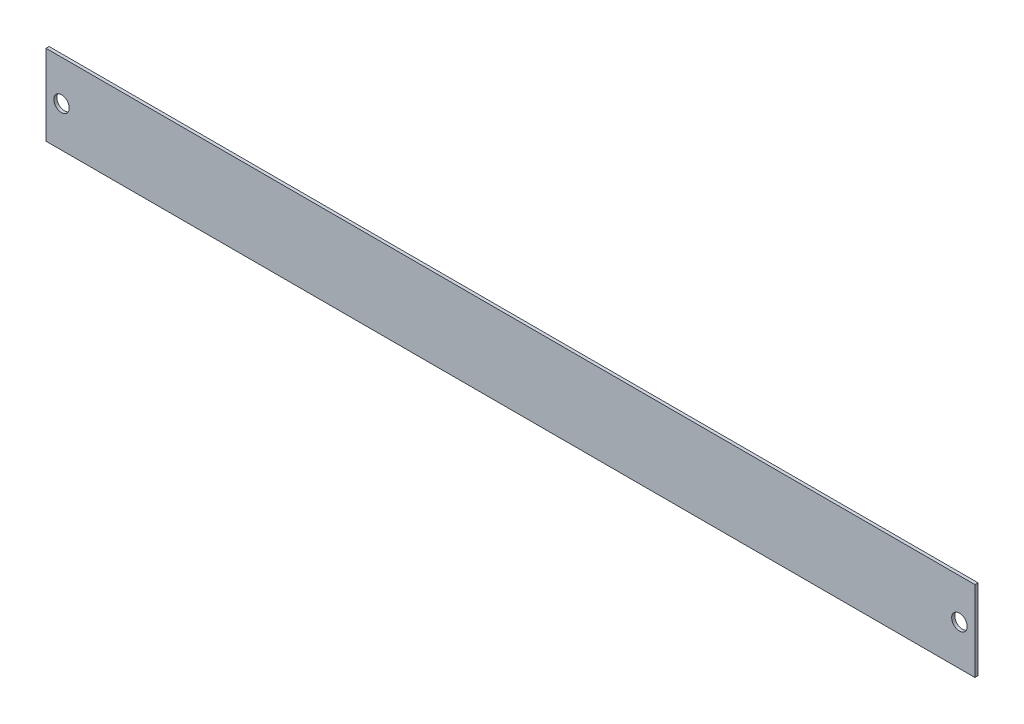
from build123d import *

# Parameters (mm, degrees)
SKETCH_1_W                = 300
SKETCH_1_H                = 26
EXTRUDE_1_DEPTH           = 1
HOLE_WIZARD_5_0_5_1_D     = 5
HOLE_WIZARD_5_0_5_1_DEPTH = 5
HOLE_WIZARD_5_0_5_1_TIP   = 1.502151548


with BuildPart() as part:
    # 草图1 → 凸台-拉伸1 (new body)
    with BuildSketch(Plane.XY):
        with Locations((0, 13)):
            Rectangle(SKETCH_1_W, SKETCH_1_H)
    extrude(amount=EXTRUDE_1_DEPTH)

    # Ø5.0 (5) 直径孔1
    with Locations(Plane.XY.offset(1)):
        with Locations((-145, 13), (145, 13)):
            Hole(HOLE_WIZARD_5_0_5_1_D / 2, depth=HOLE_WIZARD_5_0_5_1_DEPTH)
            with Locations((0, 0, -(HOLE_WIZARD_5_0_5_1_DEPTH + HOLE_WIZARD_5_0_5_1_TIP / 2))):  # 118° drill point
                Cone(0, HOLE_WIZARD_5_0_5_1_D / 2, HOLE_WIZARD_5_0_5_1_TIP, mode=Mode.SUBTRACT)


solid = part.part
